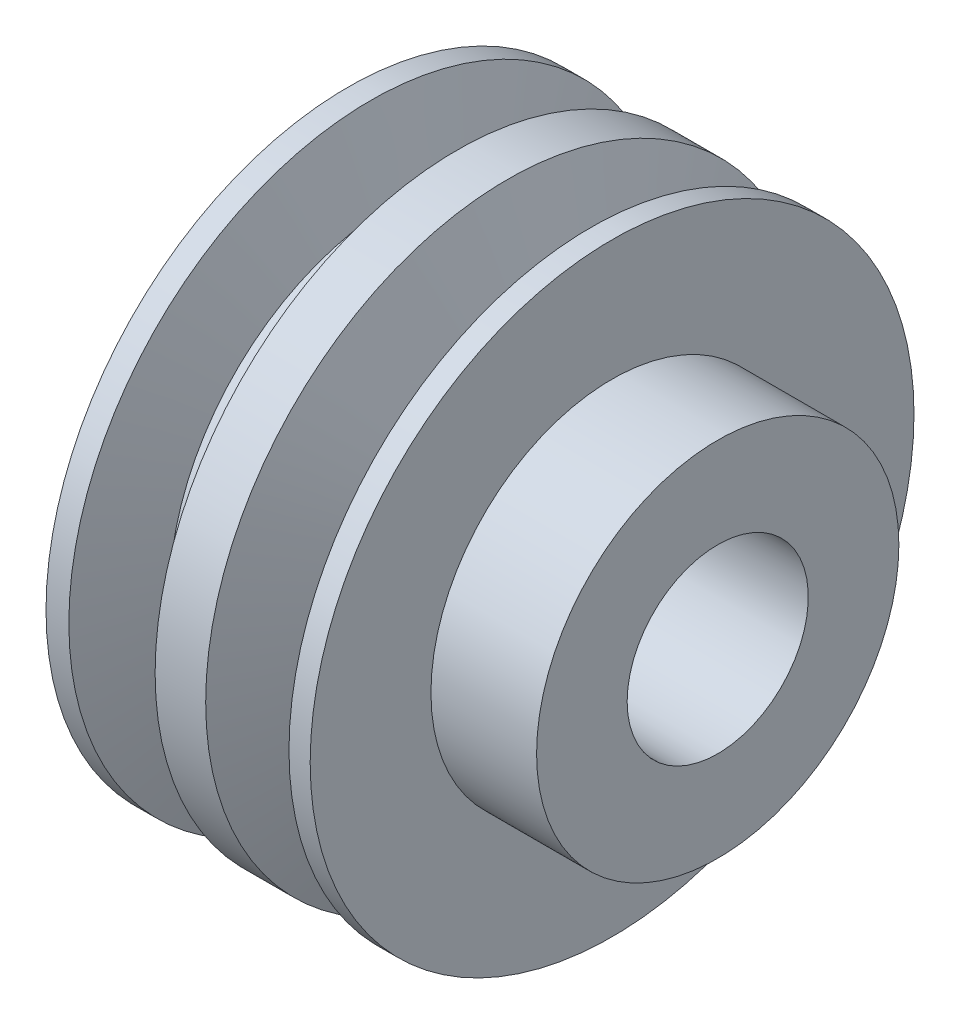
SolidWorks part; units mm, degrees
ref_plane "Front" through (0, 0, 0) normal (0, 0, 1) x (1, 0, 0)
ref_plane "Top" through (0, 0, 0) normal (0, 1, 0) x (1, 0, 0)
ref_plane "Right" through (0, 0, 0) normal (1, 0, 0) x (0, 0, -1)
sketch "Sketch1" plane through (0, 0, 0) normal (0, 1, 0) x (1, 0, 0)
  line L0 (0, 0) -> (52.0279, 0) construction
  line L1 (0, 12) -> (0, 40)
  line L2 (0, 40) -> (3.0259, 40)
  line L3 (35, 40) -> (35, 24)
  line L4 (35, 24) -> (48.9965, 24)
  line L5 (48.9965, 24) -> (48.9965, 12)
  line L7 (3.0259, 40) -> (6.4416, 30.0917)
  line L8 (6.4416, 30.0917) -> (11.8279, 30.0917)
  line L9 (11.8279, 30.0917) -> (14.4553, 40)
  line L10 (21.1553, 40) -> (25.2279, 30.0917)
  line L11 (25.2279, 30.0917) -> (28.7749, 30.0917)
  line L12 (28.7749, 30.0917) -> (32.1906, 40)
  line L13 (14.4553, 40) -> (21.1553, 40)
  line L14 (32.1906, 40) -> (35, 40)
  line L15 (0, 12) -> (48.9965, 12)
  dimension "D2" = 35
revolve "Revolve1" add sketch "Sketch1" angle 360 about L0
